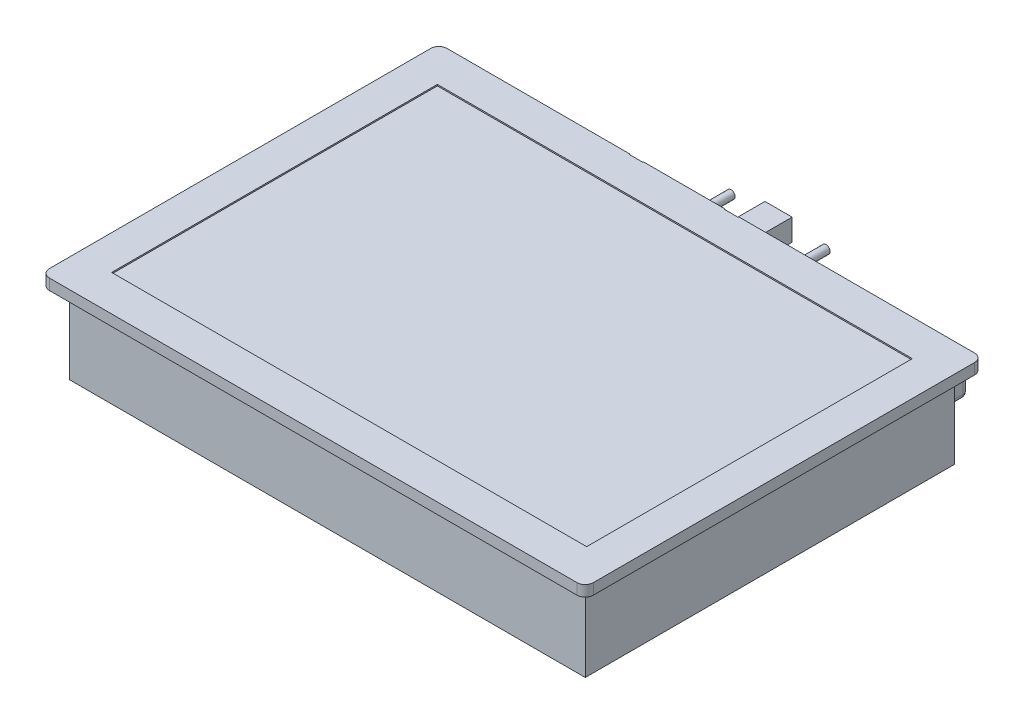
from build123d import *

# Parameters (mm, degrees)
SKETCH_1_W          = 200.4
SKETCH_1_H          = 146.5
EXTRUDE_1_DEPTH     = 17
SKETCH_2_W          = 175
SKETCH_2_H          = 120
CUT_EXTRUDE_1_DEPTH = 0.5
SKETCH_3_W          = 200.4
SKETCH_3_H          = 146.5
SKETCH_3_W_2        = 190
SKETCH_3_H_2        = 136
CUT_EXTRUDE_2_DEPTH = 30
FILLET_1_R          = 3
SKETCH_4_W          = 40
SKETCH_4_H          = 8
EXTRUDE_2_DEPTH     = 40
SKETCH_5_W          = 15
SKETCH_5_H          = 8
EXTRUDE_3_DEPTH     = 20
FILLET_2_R          = 2
SKETCH_6_R          = 1.75
EXTRUDE_4_DEPTH     = 5
CUT_EXTRUDE_3_DEPTH = 151.973640083
SKETCH_8_W          = 5
SKETCH_8_H          = 15
CUT_EXTRUDE_4_DEPTH = 151.973640083
SKETCH_9_R          = 1.5
EXTRUDE_5_DEPTH     = 35


with BuildPart() as part:
    # 草图1 → 凸台-拉伸1 (new, symmetric)
    with BuildSketch(Plane(origin=(0, 0, 0), x_dir=(1, 0, 0), z_dir=(0, 1, 0))):
        Rectangle(SKETCH_1_W, SKETCH_1_H)
    extrude(amount=EXTRUDE_1_DEPTH, both=True)

    # 草图2 → 切除-拉伸1 (cut)
    with BuildSketch(Plane(origin=(0, 17, 0), x_dir=(1, 0, 0), z_dir=(0, 1, 0))):
        Rectangle(SKETCH_2_W, SKETCH_2_H)
    extrude(amount=-CUT_EXTRUDE_1_DEPTH, mode=Mode.SUBTRACT)

    # 草图3 → 切除-拉伸2 (cut)
    with BuildSketch(Plane.XZ.offset(17)):
        Rectangle(SKETCH_3_W, SKETCH_3_H)
        Rectangle(SKETCH_3_W_2, SKETCH_3_H_2, mode=Mode.SUBTRACT)
    extrude(amount=-CUT_EXTRUDE_2_DEPTH, mode=Mode.SUBTRACT)

    # 圆角1
    fillet_1_edges = [part.edges().sort_by_distance(p)[0] for p in [
        (-100.2, 15, -73.25),
        (100.2, 15, -73.25),
        (100.2, 15, 73.25),
        (-100.2, 15, 73.25),
    ]]
    fillet(fillet_1_edges, radius=FILLET_1_R)

    # 草图4 → 凸台-拉伸2 (add)
    with BuildSketch(Plane(origin=(0, 0, -68), x_dir=(-1, 0, 0), z_dir=(0, 0, -1))):
        with Locations((9.8, -12)):
            Rectangle(SKETCH_4_W, SKETCH_4_H)
    extrude(amount=EXTRUDE_2_DEPTH)

    # 草图5 → 凸台-拉伸3 (add)
    with BuildSketch(Plane(origin=(0, 0, -68), x_dir=(-1, 0, 0), z_dir=(0, 0, -1))):
        with Locations((-72.7, -9)):
            Rectangle(SKETCH_5_W, SKETCH_5_H)
    extrude(amount=EXTRUDE_3_DEPTH)

    # 圆角2
    fillet_2_edges = [part.edges().sort_by_distance(p)[0] for p in [
        (65.2, -13, -78),
        (65.2, -5, -78),
        (80.2, -5, -78),
        (80.2, -13, -78),
        (65.2, -9, -88),
        (72.7, -5, -88),
        (80.2, -9, -88),
        (72.7, -13, -88),
    ]]
    fillet(fillet_2_edges, radius=FILLET_2_R)

    # 草图6 → 凸台-拉伸4 (add)
    with BuildSketch(Plane(origin=(0, 0, -88), x_dir=(-1, 0, 0), z_dir=(0, 0, -1))):
        with Locations((-72.7, -9)):
            Circle(SKETCH_6_R)
    extrude(amount=EXTRUDE_4_DEPTH)

    # 草图7 → 切除-拉伸3 (cut, through all)
    with BuildSketch(Plane.XZ.offset(16)):
        Polygon((-29.8, -88), (-19.8, -88), (-14.8, -98), (-14.8, -108), (-29.8, -108), align=None)
        Polygon((-4.8, -98), (-4.8, -108), (10.2, -108), (10.2, -88), (0.2, -88), align=None)
    extrude(amount=-CUT_EXTRUDE_3_DEPTH, mode=Mode.SUBTRACT)

    # 草图8 → 切除-拉伸4 (cut, through all)
    with BuildSketch(Plane.XZ.offset(16)):
        with Locations((-27.3, -80.5)):
            Rectangle(SKETCH_8_W, SKETCH_8_H)
        with Locations((7.7, -80.5)):
            Rectangle(SKETCH_8_W, SKETCH_8_H)
    extrude(amount=-CUT_EXTRUDE_4_DEPTH, mode=Mode.SUBTRACT)

    # 草图9 → 凸台-拉伸5 (add)
    with BuildSketch(Plane(origin=(0, 0, -73), x_dir=(-1, 0, 0), z_dir=(0, 0, -1))):
        with Locations(Location((27.3, -12, 0), (0, 0, 270))):
            Circle(SKETCH_9_R)
        with Locations(Location((-7.7, -12, 0), (0, 0, 270))):
            Circle(SKETCH_9_R)
    extrude(amount=EXTRUDE_5_DEPTH)


solid = part.part
